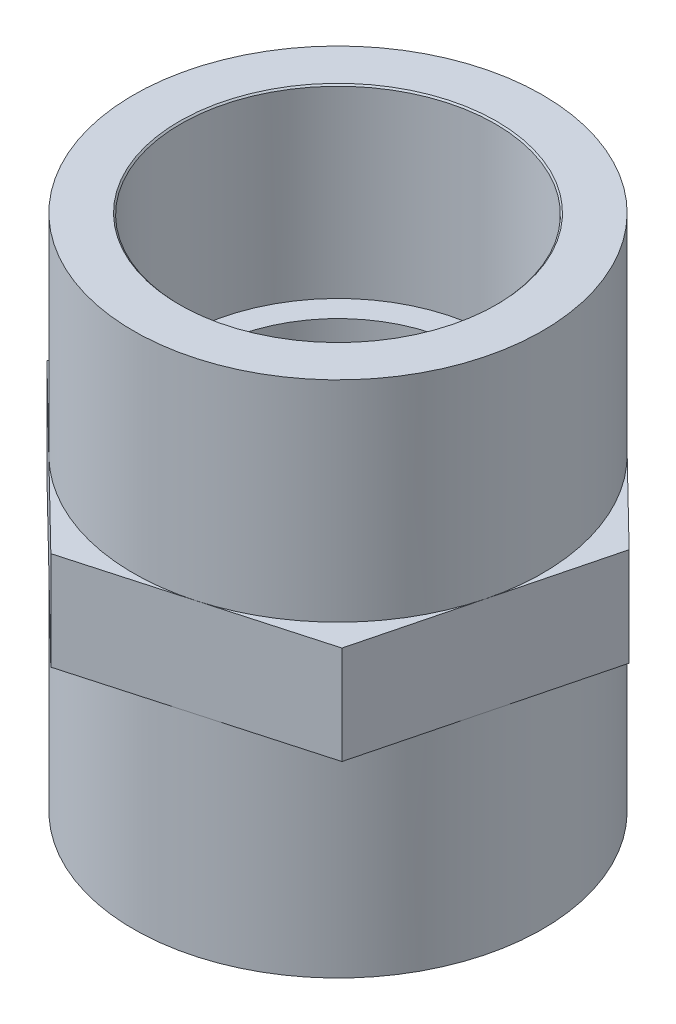
SolidWorks part; units mm, degrees
ref_plane "前视基准面" through (0, 0, 0) normal (0, 0, 1) x (1, 0, 0)
ref_plane "上视基准面" through (0, 0, 0) normal (0, 1, 0) x (1, 0, 0)
ref_plane "右视基准面" through (0, 0, 0) normal (1, 0, 0) x (0, 0, -1)
sketch "草图1" plane through (0, 0, 0) normal (0, 0, 1) x (1, 0, 0)
  line L0 (-20.8, 26.35) -> (-20.8, -26.35)
  line L1 (-20.8, -26.35) -> (0, -26.35)
  line L2 (0, -26.35) -> (0, 26.35) construction
  line L3 (0, 26.35) -> (-20.8, 26.35)
  line L4 (-16, 26.2) -> (-16, 3.7)
  line L5 (-16, 3.7) -> (-13.6, 3.7)
  line L7 (-13.6, 0) -> (-16, 0)
  line L8 (-16, 0) -> (-16, -26.35)
  line L9 (-16, 26.2) -> (-16.15, 26.35)
  dimension "D1" = 135
  dimension "H" = 52.7
  dimension "D" = 41.6
  dimension "(d2)" = 32
  dimension "(d1)" = 32.3
  dimension "D2" = 27.2
  dimension "S" = 22.5
sketch "草图2" plane through (0, 0, 0) normal (0, 0, 1) x (1, 0, 0)
  line L4 (-16, 26.2) -> (-16, 3.7) construction
  line L5 (-16, 26.2) -> (-16.15, 26.35) construction
  line L6 (-20.8, -26.35) -> (0, -26.35) construction
  line L7 (-20.8, 26.35) -> (-20.8, -26.35) construction
  line L8 (0, 26.35) -> (-20.8, 26.35) construction
  line L13 (-16, 26.2) -> (-16, -26.35)
  line L14 (-16, 26.2) -> (-16.15, 26.35)
  line L15 (-20.8, -26.35) -> (-16, -26.35)
  line L16 (-20.8, 26.35) -> (-20.8, -26.35)
  line L17 (-16.15, 26.35) -> (-20.8, 26.35)
  line L18 (0, -26.35) -> (0, 26.35) construction
  line L19 (0, -26.35) -> (0, 26.35) construction
revolve "旋转1" add sketch "草图2" angle 360 about L19
cosmetic thread "装饰螺纹线1" parameters "D1"=22.5, "D2"=32.4
sketch "草图3" plane through (0, 0, 0) normal (0, 0, 1) x (1, 0, 0)
  line L0 (0, -26.35) -> (0, 26.35) construction
  line L1 (-16, 3.7) -> (-13.6, 3.7)
  line L2 (-16, 3.7) -> (-16, 0)
  line L3 (-16, 0) -> (-13.6, 0)
  line L4 (-13.6, 3.7) -> (-13.6, 0)
  line L5 (0, -26.35) -> (0, 26.35) construction
revolve "1" add sketch "草图3" angle 360 about L5
sketch "草图4" plane through (0, 0, 0) normal (0, 1, 0) x (1, 0, 0)
  line L1 (23.1244, 6.4897) -> (5.9419, 23.2712)
  line L2 (5.9419, 23.2712) -> (-17.1824, 16.7815)
  line L3 (-17.1824, 16.7815) -> (-23.1244, -6.4897)
  line L4 (-23.1244, -6.4897) -> (-5.9419, -23.2712)
  line L5 (-5.9419, -23.2712) -> (17.1824, -16.7815)
  line L6 (17.1824, -16.7815) -> (23.1244, 6.4897)
  circle A0 centre (0, 0) radius 20.8 construction
  circle A1 centre (0, 0) radius 20.8 construction
extrude "凸台-拉伸1" add sketch "草图4" along normal mid plane 10
sketch "草图5" plane through (0, 5, 0) normal (0, 1, 0) x (1, 0, 0)
  circle A0 centre (0, 0) radius 16
extrude "切除-拉伸1" cut sketch "草图5" against normal blind 10
sketch "草图6" plane through (0, 0, 0) normal (0, 1, 0) x (1, 0, 0)
  circle A0 centre (0, 0) radius 13.5
  circle A1 centre (0, 0) radius 17.5
  dimension "D2" = 27
  dimension "D1" = 35
extrude "凸台-拉伸2" add sketch "草图6" along normal mid plane 15
